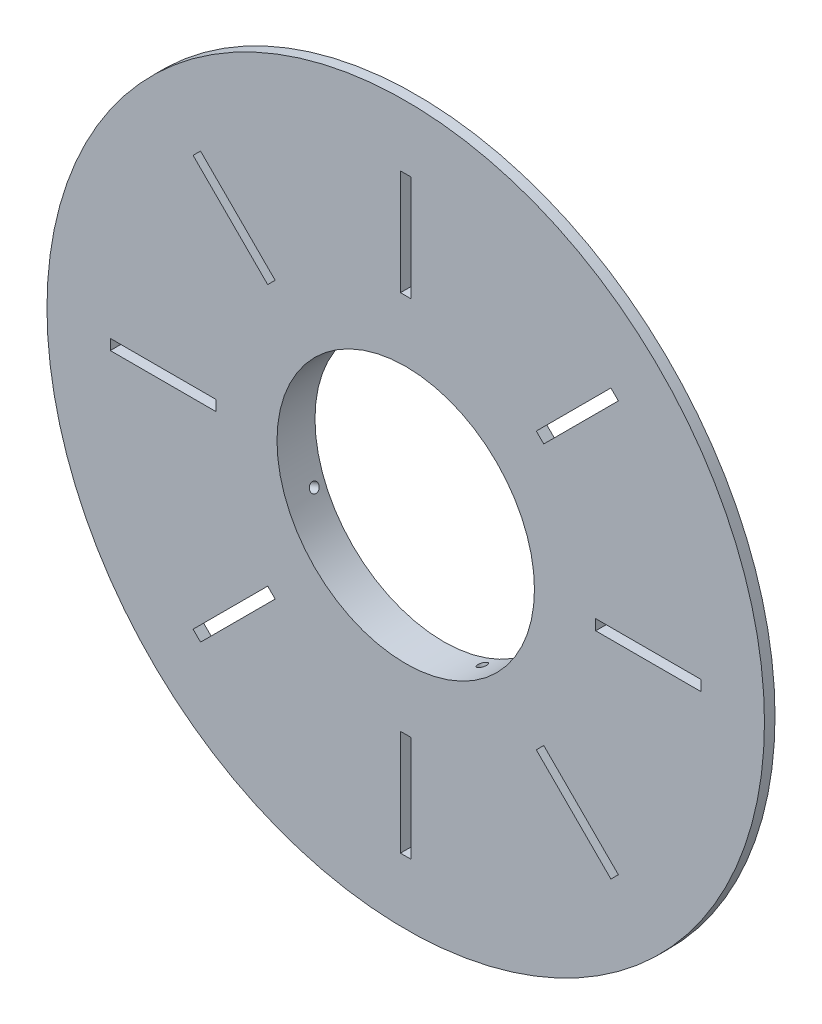
from build123d import *
from build123d.topology import SkipClean

# Parameters (mm, degrees)
SKETCH_1_R               = 170
SKETCH_1_R_2             = 61
EXTRUDE_1_DEPTH          = 2.5
SKETCH_2_W               = 5
SKETCH_2_H               = 50
CUT_EXTRUDE_1_DEPTH      = 606
PATTERN_CIRCULAR_1_COUNT = 8
EXTRUDE_START            = 13
SKETCH_3_R               = 71
SKETCH_3_R_2             = 61
EXTRUDE_2_DEPTH          = 13
PATTERN_CIRCULAR_2_COUNT = 4


with BuildPart() as part:
    # 草图1 → 凸台-拉伸1 (new, symmetric)
    with BuildSketch(Plane.XY):
        Circle(SKETCH_1_R)
        Circle(SKETCH_1_R_2, mode=Mode.SUBTRACT)
    extrude(amount=EXTRUDE_1_DEPTH, both=True)

    # 草图2 → 切除-拉伸1 (cut)
    with BuildSketch(Plane(origin=(0, 0, -2.5), x_dir=(-1, 0, 0), z_dir=(0, 0, -1))):
        with Locations((0, 115)):
            Rectangle(SKETCH_2_W, SKETCH_2_H)
    cut_extrude_1 = extrude(amount=-CUT_EXTRUDE_1_DEPTH, mode=Mode.SUBTRACT)

    # 阵列(圆周)1: 切除-拉伸1 ×8 about axis
    pattern_circular_1_axis = Axis((0, 0, 0), (0, 0, 1))
    for i in range(1, PATTERN_CIRCULAR_1_COUNT):
        add(cut_extrude_1.rotate(pattern_circular_1_axis, i * 360 / PATTERN_CIRCULAR_1_COUNT), mode=Mode.SUBTRACT)

    # 草图3 → 凸台-拉伸2 (add)
    with SkipClean():  # the faces are left unmerged after this step: merging them gives an invalid solid
        with BuildSketch(Plane(origin=(0, 0, -2.5), x_dir=(-1, 0, 0), z_dir=(0, 0, -1)).offset(EXTRUDE_START)):
            with Locations(Location((0, 0, 0), (0, 0, 180))):
                Circle(SKETCH_3_R)
            Circle(SKETCH_3_R_2, mode=Mode.SUBTRACT)
        extrude(amount=-EXTRUDE_2_DEPTH)

    # 草图4 → 切除-旋转1 (revolve, cut)
    with SkipClean():  # the faces are left unmerged after this step: merging them gives an invalid solid
        with BuildSketch(Plane(origin=(0, 0, -10.5), x_dir=(-1, 0, 0), z_dir=(0, 0, -1)), mode=Mode.PRIVATE) as cut_revolve_1_sk:
            Polygon((34.991643562, 78.728423411), (32.95910859, 79.570326962), (17.162768918, 41.434589489), (19.195303889, 40.592685937), align=None)
        cut_revolve_1 = revolve(cut_revolve_1_sk.sketch.rotate(Axis((0, 0, -10.5), (-0.38268343236509056, 0.9238795325112865, 0)), 180), axis=Axis((0, 0, -10.5), (-0.38268343236509056, 0.9238795325112865, 0)), mode=Mode.SUBTRACT)

    # 阵列(圆周)2: 切除-旋转1 ×4 about axis
    with SkipClean():  # the faces are left unmerged after this step: merging them gives an invalid solid
        pattern_circular_2_axis = Axis((0, 0, 2.5), (0, 0, -1))
        for i in range(1, PATTERN_CIRCULAR_2_COUNT):
            add(cut_revolve_1.rotate(pattern_circular_2_axis, i * 360 / PATTERN_CIRCULAR_2_COUNT), mode=Mode.SUBTRACT)


solid = part.part
